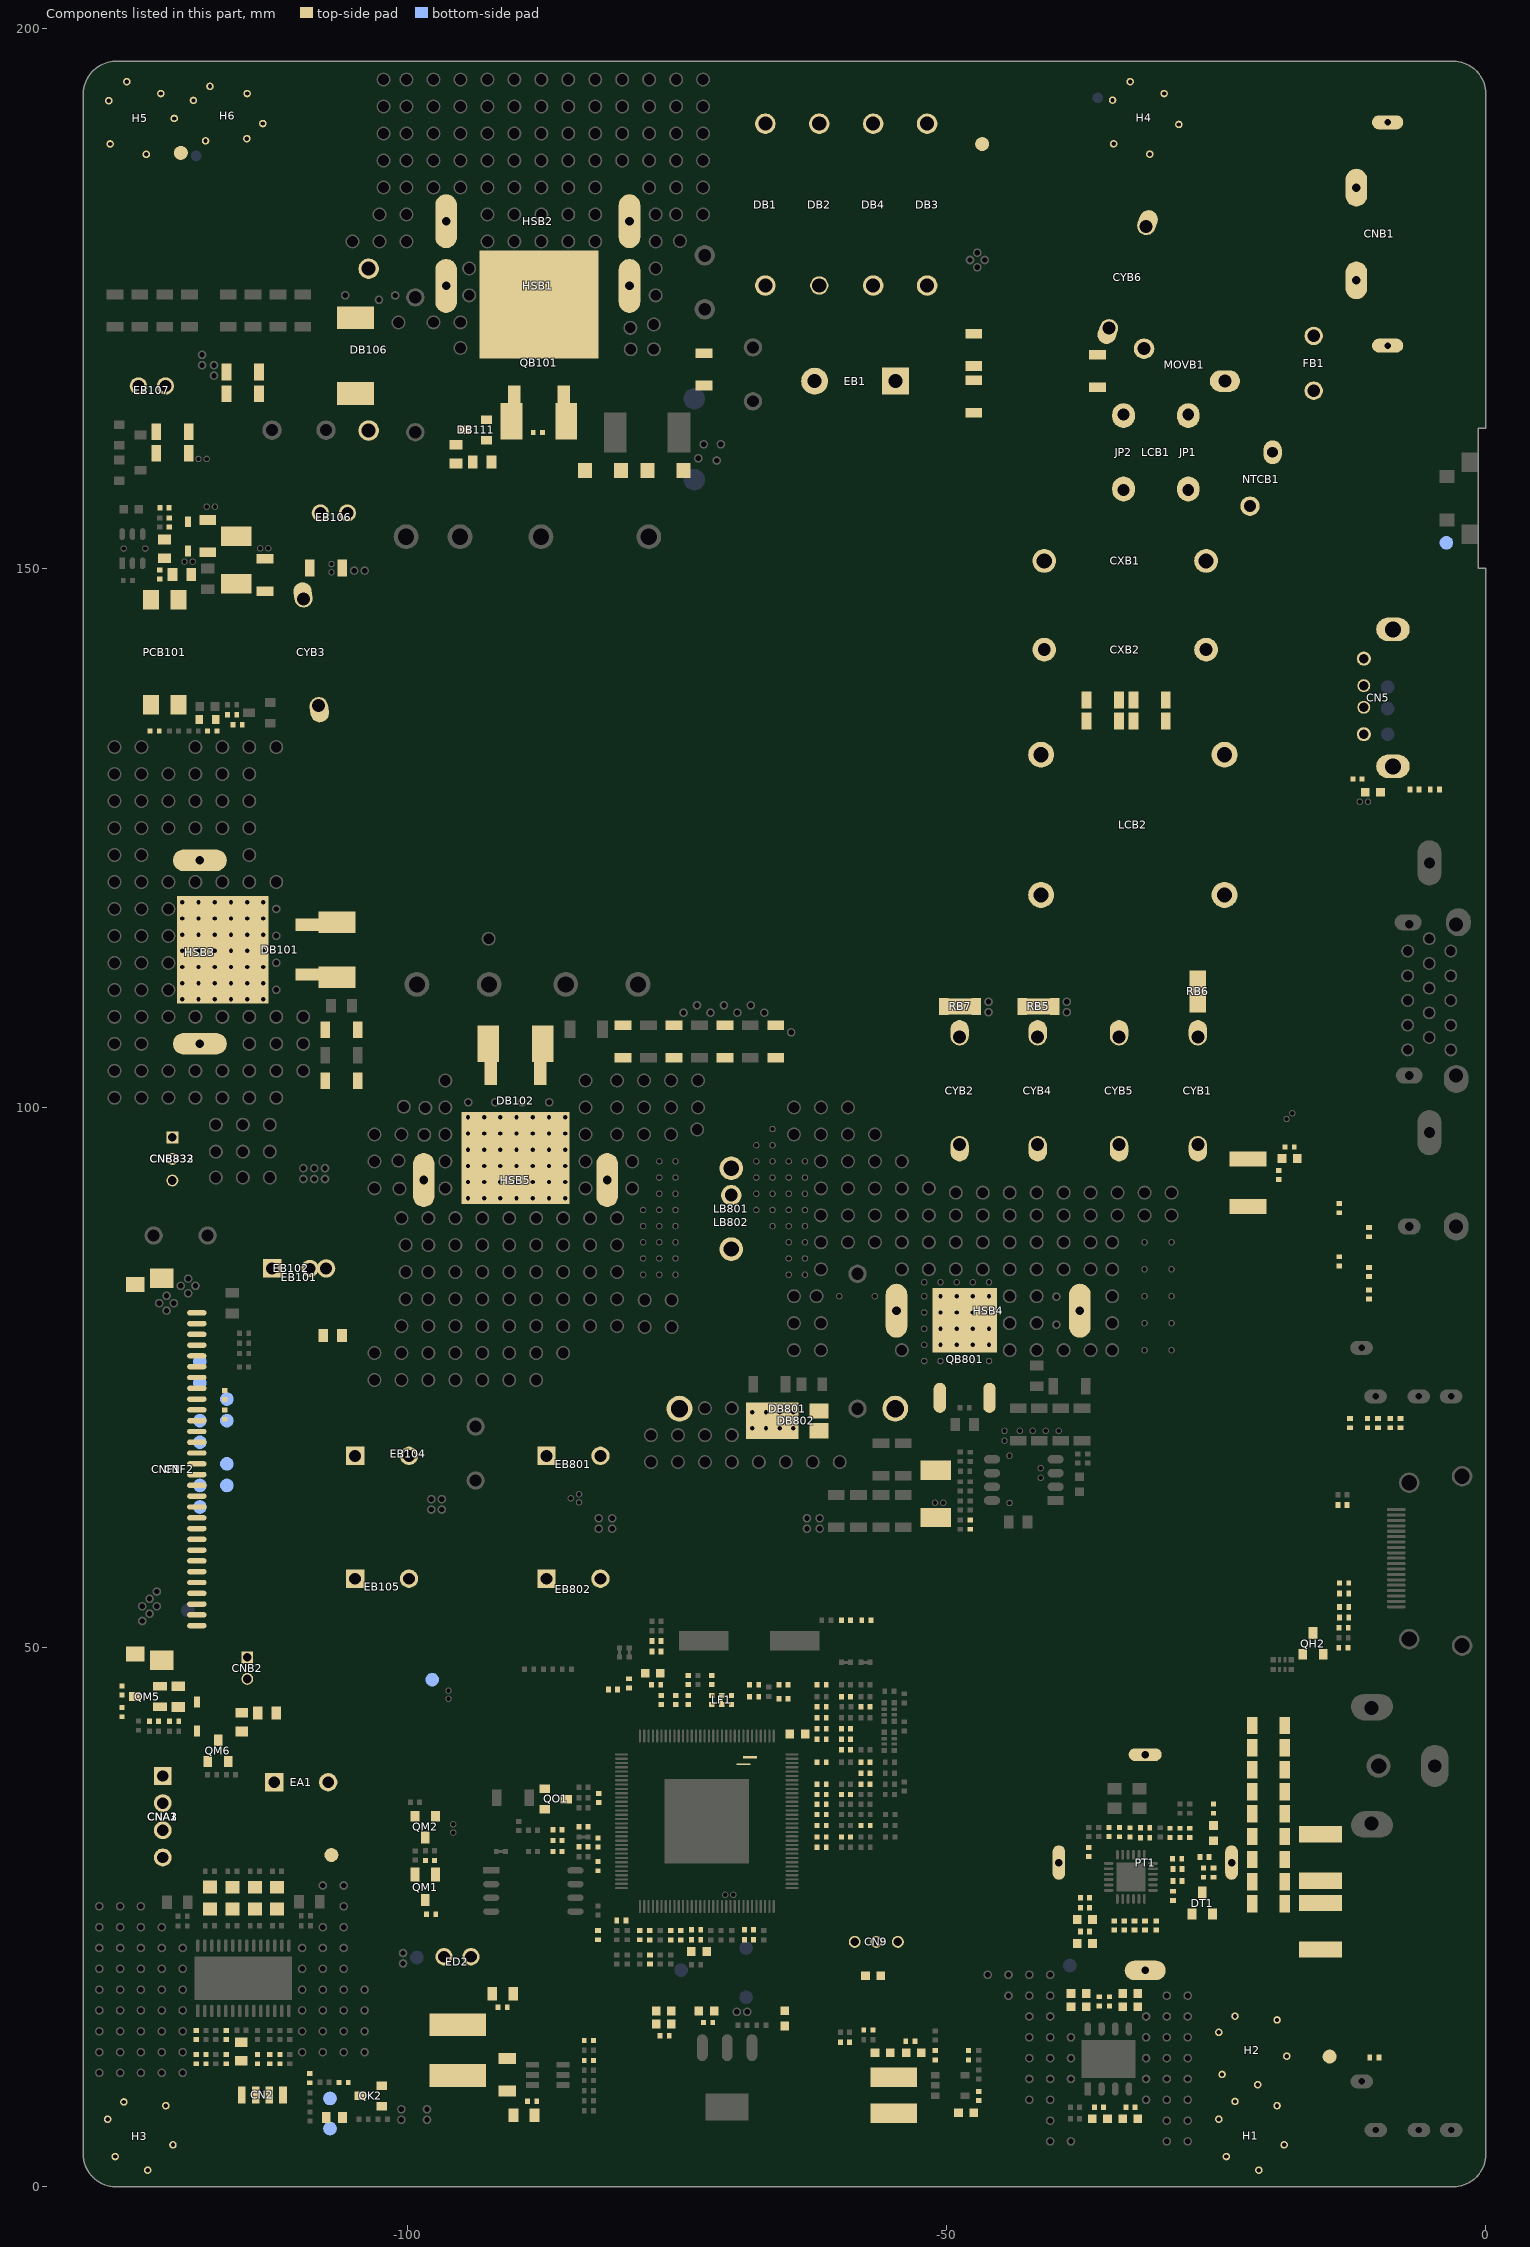
[diagram p0: the components of this part, seen from the top]
# Altium PCB MISC84438.PcbDoc (part 2 of 15)
Units mm, origin at the board's own origin, x right, y up, seen from the top; angles counter-clockwise.
Board outline 130 x 197 mm, 2 copper layers (TopLayer, BottomLayer), stack 1.571 mm thick; 574 components, 314 nets, 2636 pads, 811 vias.

## Components (designator, comment, footprint, x,y, rotation, side; value= is the part's Value field where it differs from the comment) (continued)
CB813 "100pF-0402-NPO-±5%-50V" C0402 -47.803,61.366 r90 top
CD1 "10uF-0805-X5R-±20%-16V" C0805 -89.154,6.629 r0 top
CD2 "0.1uF-0402-X5R-±20%-16V" C0402 -83.146,13.551 r0 top
CD11 "10uF-0603-X5R-±20%-6.3V" C0603 -48.171,6.858 r0 top
CD12 "NC/0.1uF-0402-X5R-±20%-16V" C0402 -47.015,8.395 r90 top
CD13 "3300pF-0402-X7R-±10%-50V" C0402 -47.955,12.179 r270 top
CD14 "10uF-0603-X5R-±20%-6.3V" C0603 -53.027,12.421 r180 top
CD15 "10uF-0603-X5R-±20%-6.3V" C0603 -55.918,12.408 r0 top
CD16 "NC/0.1uF-0402-X5R-±20%-16V" C0402 -53.34,13.487 r180 top
CD17 "Ceramic capacitor,CAP MC,6.3V,1uF,±20%,X5R,0402,SMD,TP" C0402 -51.027,12.179 r270 top
CD19 "NC/0.1uF-0402-X5R-±20%-16V" C0402 -88.392,7.925 r0 top
CD20 "NC/22pF-0402-NPO-±5%-50V" C0402 -83.146,11.697 r180 top
CD21 "NC/0.1uF-0402-X5R-±20%-16V" C0402 -91.135,16.612 r0 top
CD22 "10uF-0805-X5R-±20%-16V" C0805 -91.123,17.894 r0 top
CD41 "NC/10uF-1206-X5R-±10%-16V" C1206 -90.715,10.377 r270 top
CF1 "33pF-0402-NPO-±5%-50V" C0402 -73.939,46.964 r270 top
CF2 "0.1uF-0402-X5R-±20%-16V" C0402 -86.055,31.064 r0 top
CF4 "33pF-0402-NPO-±5%-50V" C0402 -71.755,46.964 r90 top
CF5 "10uF-0603-X5R-±20%-6.3V" C0603 -56.794,19.558 r0 top
CF6 "0.1uF-0402-X5R-±20%-16V" C0402 -82.22,36.017 r270 top
CF7 "0.1uF-0402-X5R-±20%-16V" C0402 -74.612,23.302 r90 top
CF8 "0.1uF-0402-X5R-±20%-16V" C0402 -61.57,31.445 r180 top
CF9 "0.1uF-0402-X5R-±20%-16V" C0402 -76.429,45.11 r270 top
CF10 "0.1uF-0402-X5R-±20%-16V" C0402 -61.57,36.347 r180 top
CF12 "0.1uF-0402-X5R-±20%-16V" C0402 -71.755,45.11 r270 top
CF13 "0.1uF-0402-X5R-±20%-16V" C0402 -61.57,39.344 r180 top
CF14 "0.1uF-0402-X5R-±20%-16V" C0402 -69.926,45.11 r270 top
CF15 "NC/10uF-0603-X5R-±20%-6.3V" C0603 -77.216,47.574 r180 top
CF16 "0.1uF-0402-X5R-±20%-16V" C0402 -76.911,46.507 r0 top
CF17 "0.1uF-0402-X5R-±20%-16V" C0402 -68.301,23.81 r180 top
CF18 "0.1uF-0402-X5R-±20%-16V" C0402 -78.435,23.314 r90 top
CF19 "0.1uF-0402-X5R-±20%-16V" C0402 -73.939,45.11 r270 top
CF20 "0.1uF-0402-X5R-±20%-16V" C0402 -82.296,29.705 r90 top
CF21 "0.1uF-0402-X5R-±20%-16V" C0402 -75.552,23.302 r90 top
CF22 "10uF-0603-X5R-±20%-6.3V" C0603 -72.936,21.79 r0 top
CF23 "Ceramic capacitor,CAP MC,6.3V,2.2uF,±20%,X5R,0402,SMD,TP" C0402 -75.082,45.11 r270 top
CF24 "0.1uF-0402-X5R-±20%-16V" C0402 -73.203,23.81 r180 top
CF25 "0.1uF-0402-X5R-±20%-16V" C0402 -73.203,22.872 r180 top
CF26 "0.047uF-0402-X7R-±10%-16V" C0402 -57.506,38.303 r0 top
CF28 "10uF-0603-X5R-±20%-6.3V" C0603 -63.805,41.961 r180 top
CF29 "NC/1000pF-0402-X7R-±10%-50V" C0402 -57.233,14.516 r0 top
CF30 "NC/1000pF-0402-X7R-±10%-50V" C0402 -59.405,13.398 r0 top
CF31 "NC/0.047uF-0402-X7R-±10%-16V" C0402 -57.48,33.477 r0 top
CF33 "NC/5pF-0402-NPO-±5%-50V" C0402 -116.896,71.552 r90 top
CF34 "NC/0.047uF-0402-X7R-±10%-16V" C0402 -61.57,37.312 r180 top
CF35 "NC/5pF-0402-NPO-±5%-50V" C0402 -116.896,73.381 r270 top
CF37 "10uF-0603-X5R-±20%-6.3V" C0603 -64.973,15.596 r270 top
CF38 "NC/0.1uF-0402-X5R-±20%-16V" C0402 -126.416,43.98 r270 top
CF39 "NC/NC/30pF-0402-NPO-±5%-50V" C0402 -59.309,52.489 r0 top
CF40 "Ceramic capacitor,CAP MC,50V,1000pF,±20%,X7R,0402,SMD,TP" C0402 -57.429,52.489 r180 top
CG1 "NC/0.1uF-0402-X5R-±20%-16V" C0402 -86.055,32.08 r180 top
CH8 "NC/0.1uF-0402-X5R-±20%-16V" C0402 -13.183,51.791 r0 top
CH9 "NC/0.1uF-0402-X5R-±20%-16V" C0402 -13.208,49.962 r0 top
CH10 "NC/30pF-0402-NPO-±5%-50V" C0402 -13.132,55.956 r180 top
CH15 "NC/1uF-0402-X5R-±20%-16V" C0402 -68.301,22.872 r180 top
CI1 "NC/0.047uF-0402-X7R-±10%-16V" C0402 -59.309,36.347 r0 top
CI3 "NC/0.1uF-0402-X5R-±20%-16V" C0402 -61.57,42.431 r0 top
CI4 "NC/0.1uF-0402-X5R-±20%-16V" C0402 -59.309,42.431 r0 top
CI6 "0.1uF-0402-X5R-±20%-16V" C0402 -59.309,40.5 r0 top
CI7 "0.1uF-0402-X5R-±20%-16V" C0402 -59.309,41.452 r0 top
CI8 "0.047uF-0402-X7R-±10%-16V" C0402 -57.506,37.313 r0 top
CI10 "NC/4700pF-0402-X7R-±10%-50V" C0402 -10.973,70.764 r90 top
CI11 "NC/4700pF-0402-X7R-±10%-50V" C0402 -8.865,70.764 r90 top
CK2 "0.01uF-0402-X7R-±10%-50V" C0402 -77.483,23.302 r270 top
CK4 "0.1uF-0402-X5R-±20%-16V" C0402 -109.004,10.058 r90 top
CK6 "NC/10pF-0402-NPO-±5%-50V" C0402 -83.642,31.496 r0 top
CK10 "NC/0.1uF-0402-X5R-±20%-16V" C0402 -105.867,9.652 r180 top
CL1 "NC/10uF-0603-X5R-±20%-6.3V" C0603 -72.238,16.281 r0 top
CL2 "0.1uF-0402-X5R-±20%-16V" C0402 -72.085,15.215 r0 top
CL3 "Ceramic capacitor,CAP MC,6.3V,1uF,±20%,X5R,0402,SMD,TP" C0402 -76.117,14.002 r0 top
CL4 "NC/10uF-0603-X5R-±20%-6.3V" C0603 -76.203,16.281 r0 top
CL5 "NC/10uF-0603-X5R-±20%-6.3V" C0603 -76.203,15.07 r0 top
CL6 "0.1uF-0402-X5R-±20%-16V" C0402 -35.852,7.366 r0 top
CL7 "NC/10uF-0603-X5R-±20%-6.3V" C0603 -35.776,6.299 r0 top
CL8 "NC/10uF-0603-X5R-±20%-6.3V" C0603 -32.956,6.299 r180 top
CL9 "0.1uF-0402-X5R-±20%-16V" C0402 -32.931,7.366 r180 top
CL10 "NC/0.1uF-0402-X5R-±20%-16V" C0402 -35.827,17.17 r270 top
CL11 "10uF-0603-X5R-±20%-6.3V" C0603 -37.744,17.907 r180 top
CL12 "NC/10uF-0603-X5R-±20%-6.3V" C0603 -37.744,16.688 r180 top
CL13 "NC/0.1uF-0402-X5R-±20%-16V" C0402 -34.887,17.17 r90 top
CL14 "10uF-0603-X5R-±20%-6.3V" C0603 -32.956,16.688 r0 top
CL15 "NC/10uF-0603-X5R-±20%-6.3V" C0603 -32.956,17.907 r180 top
CM1 "0.22uF-0402-X5R-±10%-16V" C0402 -97.866,30.233 r0 top
CM2 "0.1uF-0402-X5R-±20%-16V" C0402 -97.765,25.248 r180 top
CM3 "NC/0.1uF-0402-X5R-±20%-16V" C0402 -121.577,43.142 r0 top
CM4 "0.1uF-0402-X5R-±20%-16V" C0402 -126.416,45.987 r90 top
CM5 "NC/10uF-0805-X5R-±20%-16V" C0805 -121.196,45.428 r90 top
CM7 "0.022uF-0402-X7R-±10%-16V" C0402 -123.457,43.142 r180 top
CN2 "IR receiver transistor,IR Receriver,2.7-5.5V,37.9KHz,SMD,SIRAB39,SL" REMOTE-HS-1 -113.4,6.227 r0 top locked
CN5 "USB terminal,USB Jack,USB2.0,H,Single,Black,flange,Block up,DIP,103411481,VAST" USB-HD-30 -0.5,138 r90 top locked
CN9 "NC/Connector socket,connect jack,3Pin,D2.0,D,SNAP,Nature,L=2.8mm,DIP,AMA" SIP3/2.0D-3 -56.5,22.687 r0 top
CNA1 "NC/4PIN-2.54-D-H-G" SIP4/2.54D-1 -122.636,34.29 r270 top locked
CNA2 "Connector socket,connect jack,4PIN,D2.50,L,SNAP,STEP,Fool-proofing,Nature,L=3.0mm,DIP,AMA" SIP4H/2.54D-2 -122.636,34.29 r270 top locked
CNA3 "NC/Connector socket,connect jack,4Pin,D2.50,D,SNAP,nature,L=2.8mm,DIP,CNJST" SIP4/2.5D-2 -122.636,34.29 r270 top locked
CNB1 "Red-phosphorus-free connector socket,connect jack(HP),2Pin,D8.6,L,SNAP,Fool-proofing,Black,L=4.0mm,DIP,YQ" CON2-H8.6-1 -12.5,181 r90 top locked
CNB2 "Connector socket,connect jack,2Pin,D2.0,D,Beige,L=2.8mm,DIP,W2011-02SVA-SN8-ENSY,XYDT" SIP2/2.0D-1 -114.808,48.057 r270 top
CNB832 "NC/Connector socket,connect jack,3Pin,D2.0,D,SNAP,L=2.8mm,DIP,CNJST" SIP3/2.0D-CP -121.744,95.263 r270 top
CNB833 "Connector socket,connect jack,3Pin,D2.0,L,SNAP,STEP,Nature,L=2.8mm,DIP,AMA" SIP3H/2.0D-3 -121.744,95.263 r270 top
CNF1 "NC/FFC socket,FFC connector,30Pin,D1.0,Bottom,lock,SMD,F10033FA030M1WL,CT" FFC30H/1.0S-7 -122.333,66.5 r270 top
CNF2 "FFC socket,FFC connector,30Pin,D1.0,Bottom,SMD,P-TWO" FFC30H/1.0S-1 -121.111,66.5 r270 top locked
CO1 "1uF-0402-X5R-±20%-6.3V" C0402 -57.506,44.475 r0 top
CO3 "NC/1000pF-0402-X7R-±10%-50V" C0402 -61.57,43.459 r180 top
CO4 "1uF-0402-X5R-±20%-6.3V" C0402 -59.309,45.415 r180 top
CO5 "NC/1000pF-0402-X7R-±10%-50V" C0402 -61.57,44.475 r180 top
CO9 "100pF-0402-NPO-±5%-50V" C0402 -57.506,39.344 r180 top
COLD "COLD" COLD -15.494,75.794 r90 top
"Conformal Coating" "NC/Conformal coating,25kg/Can,Peters" "Conformal Coating" -147.574,131.394 r90 top
CQC "CQC" CQC -106.401,47.625 r270 top
CT1 "0.1uF-0402-X5R-±20%-16V" C0402 -36.805,31.013 r90 top
CT3 "NC/10uF-0603-X5R-±20%-6.3V" C0603 -37.16,22.543 r0 top
CT5 "0.1uF-0402-X5R-±20%-16V" C0402 -37.16,25.845 r0 top
CT6 "10uF-0603-X5R-±20%-6.3V" C0603 -37.16,24.765 r180 top
CT7 "33pF-0402-NPO-±5%-50V" C0402 -28.346,32.791 r270 top
CT8 "33pF-0402-NPO-±5%-50V" C0402 -27.432,32.791 r270 top
CT9 "0.1uF-0402-X5R-±20%-16V" C0402 -30.543,24.206 r270 top
CT10 "33pF-0402-NPO-±5%-50V" C0402 -65.107,45.212 r0 top
CT11 "0.022uF-0402-X7R-±10%-16V" C0402 -33.533,24.206 r90 top
CT12 "0.022uF-0402-X7R-±10%-16V" C0402 -34.461,24.206 r270 top
CT13 "NC/1.2pF-0402-NPO-±0.25pf-50V" C0402 -26.167,29.103 r270 top
CT14 "NC/8pF-0402-NPO-±5%-50V" C0402 -34.925,32.88 r90 top
CT15 "NC/8pF-0402-NPO-±5%-50V" C0402 -33.96,32.854 r270 top
CT17 "NC/180pF-0402-NPO-±5%-50V" C0402 -25.248,35.039 r90 top
CT18 "0.1uF-0402-X5R-±20%-16V" C0402 -37.16,26.772 r0 top
CT19 "0.022uF-0402-X7R-±10%-16V" C0402 -61.57,46.507 r180 top
CT20 "0.1uF-0402-X5R-±20%-16V" C0402 -67.825,45.415 r180 top
CT21 "0.047uF-0402-X7R-±10%-16V" C0402 -28.613,30.391 r0 top
CT23 "0.1uF-0402-X5R-±20%-16V" C0402 -67.825,46.507 r180 top
CT24 "33pF-0402-NPO-±5%-50V" C0402 -65.107,46.507 r180 top
CT25 "0.1uF-0402-X5R-±20%-16V" C0402 -29.273,32.791 r90 top
CT26 "330pF-0402-NPO-±5%-50V" C0402 -31.572,32.346 r0 top
CT27 "0.1uF-0402-X5R-±20%-16V" C0402 -32.982,32.842 r90 top
CT29 "6800pF-0402-X7R-±10%-50V" C0402 -31.572,33.274 r0 top
CT40 "Ceramic capacitor,CAP MC,1KV,470pF,±5%,NPO,1206,SMD,TP" C1206 -20.142,32.448 r180 top
CT41 "4700pF-1206-X7R-±10%-1000V" C1206 -20.142,34.569 r0 top
CT42 "4700pF-1206-X7R-±10%-1000V" C1206 -20.142,30.328 r0 top
CT43 "4700pF-1206-X7R-±10%-1000V" C1206 -20.142,28.27 r0 top
CT44 "4700pF-1206-X7R-±10%-1000V" C1206 -20.142,36.601 r0 top
CT45 "4700pF-1206-X7R-±10%-1000V" C1206 -20.142,26.213 r0 top
CT46 "4700pF-1206-X7R-±10%-1000V" C1206 -20.142,38.633 r0 top
CT47 "NC/4700pF-1206-X7R-±10%-1000V" C1206 -20.142,42.746 r0 top
CT48 "4700pF-1206-X7R-±10%-1000V" C1206 -20.142,40.691 r0 top
CU1 "NC/10uF-0603-X5R-±20%-6.3V" C0603 -10.465,129.261 r180 top
CU2 "Ceramic capacitor,CAP MC,6.3V,0.47uF,±10%,X5R,0402,SMD,TP" C0402 -11.887,130.48 r180 top
CU3 "NC/Ceramic capacitor,CAP MC,6.3V,0.47uF,±10%,X5R,0402,SMD,TP" C0402 -18.186,96.368 r0 top
CU4 "NC/10uF-0603-X5R-±20%-6.3V" C0603 -18.186,95.301 r180 top
CV1 "NC/0.047uF-0402-X7R-±10%-16V" C0402 -61.57,34.493 r0 top
CV3 "NC/0.047uF-0402-X7R-±10%-16V" C0402 -61.57,33.477 r0 top
CV7 "NC/0.047uF-0402-X7R-±10%-16V" C0402 -59.309,32.41 r0 top
CV9 "NC/33pF-0402-NPO-±5%-50V" C0402 -61.57,32.41 r180 top
CV10 "NC/33pF-0402-NPO-±5%-50V" C0402 -61.57,35.433 r180 top
CXB1 "X capacitor,CAP X2,MP,275VAC,0.47uF,±10%,S,15mm-Mini,PC,DIP,BM" CAP18*8.5-V-15 -33.432,150.692 r180 top locked
CXB2 "NC/X capacitor,CAP X2,MP,280VAC,0.1uF,±10%,P,15mm,PC,DIP,JH" CAP18*5*11.5-V-15 -33.432,142.471 r0 top
CYB1 "Y capacitor,CAP Y1,CD,470pF,400VAC,±20%,KS,10mm,Y5U,DIP,Walsin" CAP13*5-V-10-1 -26.691,101.582 r270 top locked
CYB2 "Y capacitor,CAP Y1,CD,470pF,400VAC,±20%,KS,10mm,Y5U,DIP,Walsin" CAP13*5-V-10-1 -48.777,101.582 r270 top
CYB3 "Y capacitor,CAP Y1,CD,470pF,400VAC,±20%,KS,10mm,Y5U,DIP,Walsin" CAP13*5-V-10-1 -108.882,142.227 r278 top locked
CYB4 "NC/Y capacitor,CAP Y1,CD,47pF,400VAC,±5%,KS,10mm,SL,DIP,BULK,Walsin" CAP13*5-V-10-1 -41.538,101.582 r270 top locked
CYB5 "NC/Y capacitor,CAP Y1,CD,47pF,400VAC,±5%,KS,10mm,SL,DIP,BULK,Walsin" CAP13*5-V-10-1 -33.994,101.582 r270 top locked
CYB6 "Y capacitor,CAP Y1,CD,100pF,400VAC,±10%,KS,10mm,Y5P,DIP,Walsin" CAP13*5-V-10-1 -33.2,177 r70 top
DB1 "Rectifier diode,DIO SI S,2.5A,1000V,DO-15,DIP,RL257G,YJ" D2-H-15#1 -66.788,183.722 r90 top locked
DB2 "Rectifier diode,DIO SI S,2.5A,1000V,DO-15,DIP,RL257G,YJ" D2-H-15#2 -61.788,183.722 r270 top locked
DB3 "Rectifier diode,DIO SI S,2.5A,1000V,DO-15,DIP,RL257G,YJ" D2-H-15#3 -51.788,183.722 r90 top locked
DB4 "Rectifier diode,DIO SI S,2.5A,1000V,DO-15,DIP,RL257G,YJ" D2-H-15#4 -56.788,183.722 r270 top locked
DB101 "Schottky diode,DIO SBD D1,10A,150V,TO-263,SMD,HBR10150SS,JLHW" D2PAK3#1 -117.091,114.655 r90 top locked
DB102 "Schottky diode,DIO SBD D1,10A,200V,TO-263,SMD,HBR10200SS,JLHW" D2PAK3#1 -89.948,95.345 r180 top
DB103 "NC/Rectifier diode,DIO SI S,3A,1000V,SMC,SMD,HS3M R6,TSC" DIODE-SMC -104.775,169.723 r90 top locked
DB104 "Rectifier diode,DIO SI S,1A,1000V,SMAF,SMD,M7F,YJ" DIODE-S-2 -115.83,150.795 r90 top
DB106 "Rectifier diode,DIO FRD S,2A,1000V,DO-15,DIP,FR207G-FG-WS,WILLAS" D2-H-15#5 -103.554,170.282 r270 top
DB109 "Rectifier diode,DIO FRD S,1.2A,800V,SOD-123FL,SMD,F1K,YJ" DIODE-S-14 -81.842,159.075 r180 top
DB110 "Rectifier diode,DIO FRD S,1.2A,800V,SOD-123FL,SMD,F1K,YJ" DIODE-S-14 -76.028,159.075 r180 top
DB111 "Switching diode,DIO SW D1,215mA,85V,SOT-23,SMD,KAV70,KEXIN" SO-23 -93.637,162.839 r270 top
DB112 "NC/Switching diode,DIO SW S,200mA,250V,SOD-323,SMD,BAV21WS,BLUE ROCKET" DIODE-S-12 -120.307,152.971 r270 top
DB801 "Schottky diode,DIO SBD S,3A,100V,DO-201AD,DIP,SR3100,YJ" D3-H-20-2 -64.742,72.114 r180 top
DB802 "NC/TSPB5H150S" DIODE-S-13 -64.734,70.989 r90 top
DB804 "Rectifier diode,DIO SI S,1A,1000V,SMAF,SMD,M7F,YJ" DIODE-S-2 -50.99,64.224 r270 top
DH2 "NC/0ohm-0402-±5%-1/16W" DIODE-S0402 -13.284,63.195 r0 top
DH3 "NC/NC/AVLC18S02003" DIODE-S0402 -13.132,54.991 r0 top
DH6 "NC/NC/AVLC18S02003" DIODE-S0402 -13.132,53.746 r0 top
DH7 "NC/NC/AVLC18S02003" DIODE-S0402 -13.132,52.756 r0 top
DH8 "NC/NC/AVLC18S02003" DIODE-S0402 -80.137,24.689 r0 top
DH9 "NC/NC/AVLC18S02003" DIODE-S0402 -82.296,23.314 r90 top
DI1 "NC/AVLC18S02003" DIODE-S0402 -10.82,82.702 r90 top
DI2 "NC/AVLC18S02003" DIODE-S0402 -10.82,88.468 r90 top
DI3 "NC/AVLC18S02003" DIODE-S0402 -13.589,90.703 r90 top
DI5 "NC/AVLC18S02003" DIODE-S0402 -10.338,11.989 r180 top
DK1 "TVS diode,DIO ESD,3pF,58V,0402,SMD,SDV1005H260C030YPTF,Sunlord" DIODE-S0402 -77.495,21.054 r270 top
DK20 "WEJT61RC-871-red" DIODE-S0603 -106.73,6.417 r0 top locked
DM1 "NC/Switching diode,DIO SW S,150mA,75V,SOD-323,SMD,1N4148WS,BLUE ROCKET" DIODE-S-12 -119.456,43.586 r90 top
DO1 "NC/AVLC18S02003" DIODE-S0402 -10.008,70.764 r90 top
DO2 "NC/AVLC18S02003" DIODE-S0402 -12.573,70.764 r90 top
DO3 "NC/AVLC18S02003" DIODE-S0402 -7.899,70.764 r90 top
DT1 "Switching diode,DIO SW D2,75V,SOT-23,SMD,KAV99,KEXIN" SO-23 -26.289,26.289 r180 top
DT2 "NC/AVLC18S02003" DIODE-S0402 -76.879,50.569 r0 top
DT3 "NC/AVLC18S02003" DIODE-S0402 -76.879,49.603 r0 top
DU1 "NC/" DIODE-S0402 -80.899,46.101 r0 top
DU2 "NC/" DIODE-S0402 -79.426,46.66 r270 top
DU3 "NC/" DIODE-S0402 -6.604,129.488 r0 top
DU4 "NC/" DIODE-S0402 -4.724,129.488 r180 top
DV1 "NC/NC/AVLC18S02003" DIODE-S0402 -13.589,85.776 r90 top
DV2 "NC/NC/AVLC18S02003" DIODE-S0402 -10.82,84.785 r90 top
E0N "TEST" TP -119.2,63 r180 bottom
E0P "TEST" TP -119.2,65 r180 bottom
E1N "TEST" TP -116.7,65 r180 bottom
E1P "TEST" TP -116.7,67 r180 bottom
E2N "TEST" TP -119.2,69 r180 bottom
E2P "TEST" TP -119.2,71 r180 bottom
E3N "TEST" TP -119.2,74.5 r180 bottom
E3P "TEST" TP -119.2,76.5 r180 bottom
EA1 "Aluminum electrolytic capacitor,CAP AL,16V,470uF,±20%,KM,P,5.0mm,10×12.5,DIP,TP,Samxon" EC(10*12.5)-V-5#1 -109.804,37.486 r0 top locked
EB1 "Aluminum electrolytic capacitor,CAP AL,450V,82uF,±20%,SL,KL,BK,7.5mm,18×35.5,DIP,CapXon" EC(18*41)-H-7.5-1 -58.458,164.859 r0 top locked
EB101 "Aluminum electrolytic capacitor,CAP AL,25V,470uF,±20%,LD,GK,P,5.0mm,10×12.5,DIP,TP,Samxon" EC(10*12.5)-V-5#2 -110,85.114 r0 top locked
EB102 "NC/270uF-16V-±20%-8×11-105℃-RP-short leg-F=3.5(Elite)" EC(8*11)-V-3.5 -110.75,85.114 r0 top locked
EB104 "Aluminum electrolytic capacitor,CAP AL,63V,100uF,±20%,LD,GF,P,5.0mm,10×12.5,DIP,TP,CapXon" EC(10*12.5)-V-5#3 -102.311,67.742 r0 top locked
EB105 "Aluminum electrolytic capacitor,CAP AL,63V,100uF,±20%,LD,GF,P,5.0mm,10×12.5,DIP,TP,CapXon" EC(10*12.5)-V-5#4 -102.311,56.35 r0 top locked
EB106 "Aluminum electrolytic capacitor,CAP AL,50V,10uF,±20%,LF,GH,P,2.5mm,5×11,DIP,TP,CapXon" EC(5*11)-V-2.5#1 -106.782,155.138 r0 top locked
EB107 "NC/Aluminum electrolytic capacitor,CAP AL,50V,4.7uF,±20%,LC,LL,P,2.5mm,5×11,DIP,TP,CapXon" EC(5*11)-V-2.5#2 -123.652,166.916 r0 top locked
EB801 "Aluminum electrolytic capacitor,CAP AL,100V,47uF,±20%,LD,SF,P,5.0mm,10×12.5,DIP,TP,Samxon" EC(10*12.5)-V-5#5 -84.573,67.742 r0 top locked
EB802 "NC/47uF-100V-±20%-10×12-105℃-EV-taped reel-F=5.0(Elite)" EC(10*12.5)-V-5#6 -84.573,56.35 r0 top locked
ECN "TEST" TP -116.7,71 r180 bottom
ECP "TEST" TP -116.7,73 r180 bottom
ED2 "Aluminum electrolytic capacitor,CAP AL,10V,470uF,±20%,KM,P,2.5mm,6.3×11.0,DIP,TP,Samxon" EC(6.3*11)-V-2.5 -95.326,21.311 r0 top locked
F1 "NC/MSMD110" FUSE3.5A-S -22.041,93.059 r270 top
F2 "0ohm-0402-±5%-1/16W" R0402 -19.196,93.777 r90 top
FB1 "Slow-blow fuse,FUSE T,P,3.15A,250VAC,8.5×4.0×8mm,DIP,TP,Walter" "FUSE8.5*4-V-5(T3.15AL 250V~)" -15.953,169.012 r90 top
GDT1 "NC/Gas discharge tube,GDT,700V,2000A,TP,4.5*3.2mm,SMD,4532-091-LF,Brightking" SMD4532-1 -15.316,30.505 r270 top
GDT2 "NC/Gas discharge tube,GDT,700V,2000A,TP,4.5*3.2mm,SMD,4532-091-LF,Brightking" SMD4532-1 -15.316,24.143 r90 top
GL1 "Silicone,0.5g,general,60,white,SLD-8854W,XY" "Silica gel-20" -48.006,132.461 r180 top
H1 "Location hole" ASSE4.0C-3#1 -22,5 r0 top locked
H2 "Location hole" ASSE4.0C-3#2 -22,13 r0 top locked
H3 "Location hole" ASSE4.0C-3#3 -125,5 r0 top locked
H4 "Location hole" ASSE4.0C-3#4 -32,192 r0 top locked
H5 "Location hole" ASSE4.0C-3#5 -125,192 r0 top locked
H6 "Location hole" ASSE4.0C-3#6 -117,192 r0 top locked
"High Voltage" "High Voltage" "High Voltage" -21.59,177.971 r0 top
HOT "HOT" HOT -38.964,113.64 r0 top
HS1 "Heatsink,6-series aluminium alloy,14.0×14.0×6.0mm,natural colour,XXWJ" HS(14*14*6) -72.212,33.871 r0 top locked
HSB1 "NC/17.5×14.5×0.5- natural finish -Cu-MRD" HS038 -87.874,176.188 r180 top
HSB2 "NC/17.5×14.5×0.5- natural finish -Cu-MRD" HS038 -87.874,182.188 r180 top
HSB3 "NC/17.5×14.5×0.5- natural finish -Cu-MRD" HS038 -119.2,114.438 r270 top
HSB4 "NC/17.5×14.5×0.5- natural finish -Cu-MRD" HS038 -46.126,81.193 r0 top
HSB5 "NC/17.5×14.5×0.5- natural finish -Cu-MRD" HS038 -89.948,93.305 r180 top
IR "TEST" TP -107.137,5.385 r180 bottom
JP1 "NC/Jumper,RES JUMP,0.6,7.0mm,DIP" JP7.0#1 -27.582,160.763 r90 top locked
JP2 "NC/Jumper,RES JUMP,0.6,7.0mm,DIP" JP7.0#2 -33.582,160.763 r90 top locked
KEY "TEST" TP -3.658,152.375 r180 bottom
LB801 "Differential-mode inductor,Inductor,DR12×12,70uH,0.15×12P,38.5Ts,H13.5MAX,SYDR1212-L070uA,DIP,DL" L/LC2/15*14.5-V7.5 -69.946,90.65 r90 top locked
LB802 "NC/Differential-mode inductor,Inductor,DR12×14,68uH,0.45,20Ts,H13.5MAX,SYDR1214-L068uA,DIP,Soldier" L(13.5*15.5)-V-5 -69.945,89.4 r90 top locked
LBA1 "Ferrite bead,BEAD,300ohm,0805,3000mA,SMD,TP,HCB2012KF-301T30,Tai-tech" L0805 -118.274,26.759 r90 top
LBA2 "Ferrite bead,BEAD,300ohm,0805,3000mA,SMD,TP,HCB2012KF-301T30,Tai-tech" L0805 -116.191,26.733 r90 top
LBA3 "Ferrite bead,BEAD,300ohm,0805,3000mA,SMD,TP,HCB2012KF-301T30,Tai-tech" L0805 -114.108,26.733 r90 top
LBA4 "Ferrite bead,BEAD,300ohm,0805,3000mA,SMD,TP,HCB2012KF-301T30,Tai-tech" L0805 -112.051,26.733 r90 top
LCB1 "Common-mode choke,Common Choke,T9×5×3,230uH MIN,0.45×1P,7.5Ts,H14.0MAX,SYT09-L230uA,DIP,CK" L/LC4/12.8*10-V-6*7 -30.582,160.763 r180 top locked
LCB2 "Common-mode choke,Common Choke,UC1614,10.5mH±10%,0.15×1.0mm,48Ts,H14.0MAX,SYUC16-L10.5mA,DIP,CH" L/LC4/21*17-H-17*13 -32.722,126.231 r180 top locked
LD2 "Power inductor,Power Inductor,6.8uH,±20%,1.3A,0.23×1P,DR4.5×3.2,SMD,DSB4532-6R8M-LF,BLDX" L(4.5*3.5)-S -54.864,8.471 r90 top
LD3 "Power inductor,Power Inductor,4.7uH,±20%,2.8A,0.32×1P,DR5.8×4.5,SMD,PIO54-4R7MTP02,FH" L(6.0*4.5)-S -95.301,12.649 r90 top
LED "TEST" TP -107.137,8.179 r180 bottom
LF1 "NC/0ohm-0402-PCB" R0402SC -70.841,45.11 r90 top
LF6 "0ohm-0402-±5%-1/16W" R0402 -61.57,41.453 r180 top
LT1 "Multilayer inductor,HF Inductor,68nH,±5%,0402,SMD,SDCL1005C68NJTDF,Sunlord" L0402 -31.61,24.206 r90 top
LT2 "GZ1005U102CTF(1000ohm-300mA)" L0402 -32.575,24.206 r270 top
LT3 "0ohm-0402-±5%-1/16W" L0402 -25.227,29.103 r270 top
LT6 "GZ1005U102CTF(1000ohm-300mA)" L0402 -28.981,26.962 r270 top
LT8 "GZ1005U102CTF(1000ohm-300mA)" L0402 -28.588,28.32 r0 top
LT9 "NC/SDCL1608CR22JT(F)" L0603 -25.248,32.779 r90 top
LT10 "SDCL1005CR18JTDF(180nH-0402±5%-C)" L0402 -28.588,29.425 r0 top
LT11 "NC/SDCL1005CR27JTDF (Sunlord)" L0402 -26.086,30.556 r180 top
LT12 "Ferrite bead,BEAD,120ohm,0402,500mA,SMD,TP,GZ1005U121CTF,Sunlord" L0402 -37.16,23.66 r0 top
M1 "MARK" MARK -14.478,12.052 r0 top
M2 "MARK" MARK -107.01,30.734 r0 top
M3 "MARK" MARK -120.968,188.519 r0 top
M4 "MARK" MARK -46.685,189.332 r0 top
Manufacture_Info "Manufacture_Info" Manufacture_Info -73.4,33.6 r180 top
MOVB1 "Varistor,VARISTOR,128J,680V,4000A,S,7.5mm,10mm,DIP,Thinking" VR(13*5)-V-7.5 -27.932,168.866 r0 top
"NO DOLBY" "NO DOLBY" "NO DOLBY-SILK" -80.5,5.9 r0 bottom
NTCB1 "SCK102R55AMBY502 (short leg / Weiqin)" NTC(10*5)-V5 -20.812,158.268 r90 top
PCB101 "LTV-817S-TA-B (Lite-On)" OC4-S-1 -122.45,142.227 r0 top locked
PT1 "20.3×16.3×6-LHD (with sealing)" SHIELD(16*20*6) -31.572,20.041 r0 top locked
PWM_REF "NC/TEST" TP_BL -97.663,46.99 r90 bottom
QB101 "MOSFET,NMOS,7A,650V,0.55ohm@ID=3.5A@VGS=10V,TO-252,LSG65R650HT,LONTEN" D2PAK3#2 -87.871,171.12 r270 top
QB801 "MOSFET,NMOS,15A,100V,0.105ohm@ID=6A@VGS=10V,TO-252,PA110BDA,UNIKC" TO-252-GDS -48.311,80.315 r0 top locked
QH2 "LMBT3904LT1G" SOT-23 -16.027,50.368 r180 top
QK2 "NC/MMBT3904(f≥350MHz)" SOT-23 -103.365,8.407 r270 top
QM1 "MOSFET,PMOS,-4.2A,-30V,0.052ohm@ID=-4.2A@VGS=-10V,SOT23-3,AO3401,BLUE ROCKET" SOT-23-1 -98.311,27.731 r0 top
QM2 "MMBT3904(f≥350MHz)" SOT-23 -98.311,33.319 r0 top
QM5 "MOSFET,PMOS,-4.3A,-30V,0.078ohm@ID=-3A@VGS=-4.5V,SOT-23,AO3487,AOS" SOT-23-1 -124.092,45.428 r270 top
QM6 "MMBT3904(f≥350MHz)" SOT-23 -117.526,40.411 r180 top
QO1 "NC/MMBT3904(f≥350MHz)" SOT-23 -86.208,35.938 r90 top
R1 "4K7ohm-0402-±5%-1/16W" R0402 -83.642,33.35 r180 top
R2 "4K7ohm-0402-±5%-1/16W" R0402 -82.296,31.902 r90 top
R3 "NC/4K7ohm-0402-±5%-1/16W" R0402 -86.055,33.071 r180 top
R5V "NC/0ohm-0805-±5%-1/8W" R0805 -112.979,43.917 r180 top
R12V "0ohm-0805-±5%-1/8W" R0805 -115.316,43.053 r90 top
RA1 "4K7ohm-0402-±5%-1/16W" R0402 -119.544,11.822 r270 top
RA2 "NC/" GND#1 -68.223,39.802 r180 top
RA3 "10ohm-0805-±5%-1/8W" R0805 -115.367,12.522 r90 top
RA4 "NC/100Kohm-0402-±5%-1/16W" R0402 -116.737,11.822 r270 top
RA5 "1Kohm-0402-±5%-1/16W" R0402 -111.772,11.822 r90 top
RA8 "4K7ohm-0402-±5%-1/16W" R0402 -119.544,14.057 r90 top
RA11 "4K7ohm-0402-±5%-1/16W" R0402 -113.854,11.822 r90 top
RA12 "NC/3K3ohm-0402-±5%-1/16W" R0402 -112.737,11.822 r90 top
RA14 "NC/0ohm-0402-±5%-1/16W" R0402 -116.737,14.057 r90 top
RA15 "NC/" GND#2 -68.809,39.167 r180 top
RA21 "1Kohm-0402-±5%-1/16W" R0402 -118.629,11.822 r90 top
RB1 "1M2ohm-1206-±5%-1/4W" R1206 -31.168,137.812 r180 top
RB2 "1M2ohm-1206-±5%-1/4W" R1206 -31.168,135.851 r180 top
RB3 "1M2ohm-1206-±5%-1/4W" R1206 -35.511,137.811 r180 top
RB4 "1M2ohm-1206-±5%-1/4W" R1206 -35.511,135.849 r180 top
RB5 "NC/0ohm-1206-PCB-D" R1206SC -41.47,109.398 r180 top
RB6 "NC/0ohm-1206-PCB-D" R1206SC -26.7,110.8 r270 top
RB7 "NC/0ohm-1206-PCB-D" R1206SC -48.734,109.398 r180 top
RB8 "30ohm-1206-±5%-1/4W" R1206 -36,168.3 r90 top
RB101 "330Kohm-1206-±5%-1/4W" R1206 -47.473,170.256 r270 top
RB102 "330Kohm-1206-±5%-1/4W" R1206 -47.473,165.938 r270 top
RB103 "Thick-film resistor,RES,1/16W,3.6Kohm,±1%,0402,SMD" R0402 -122.022,154.254 r90 top
RB104 "Thick-film resistor,RES,1/16W,39Kohm,±1%,0402,SMD" R0402 -122.936,149.428 r270 top
RB105 "Thick-film resistor,RES,1/16W,510ohm,±1%,0402,SMD" R0402 -122.479,155.613 r0 top
RB106 "Thick-film resistor,RES,1/8W,68ohm,±5%,0805,SMD" R0805 -93.04,159.88 r0 top
RB107 "Thick-film resistor,RES,1/8W,20ohm,±5%,0805,SMD" R0805 -95.462,160.596 r90 top
RB109 "Thick-film resistor,RES,1/16W,10Kohm,±1%,0402,SMD" R0402 -87.871,162.598 r180 top
RB110 "0ohm-1206-±5%-1/4W" R1206 -121.742,160.68 r0 top
RB111 "0ohm-1206-±5%-1/4W" R1206 -121.742,162.655 r0 top
RB112 "NC/33Kohm-0805-±1%-1/8W" R0805 -122.479,151.816 r270 top
RB113 "Thick-film resistor,RES,1/8W,300Kohm,±1%,0805,SMD" R0805 -120.879,149.428 r0 top
RB114 "Thick-film resistor,RES,1/4W,4.7ohm,±1%,1206,SMD" R1206 -113.16,149.395 r90 top
RB116 "NC/10ohm-1206-±5%-1/4W" R1206 -118.478,152.984 r90 top
RB117 "Thick-film resistor,RES,1/4W,10ohm,±5%,1206,SMD" R1206 -115.222,166.201 r180 top
RB118 "Thick-film resistor,RES,1/4W,10ohm,±5%,1206,SMD" R1206 -115.222,168.205 r180 top
RB119 "Thick-film resistor,RES,1/4W,10ohm,±5%,1206,SMD" R1206 -72.477,168.453 r90 top
RB124 "68ohm-1206-±5%-1/4W" R1206 -65.813,106.143 r270 top
RB125 "68ohm-1206-±5%-1/4W" R1206 -70.533,106.142 r270 top
RB126 "68ohm-1206-±5%-1/4W" R1206 -75.253,106.142 r270 top
RB127 "68ohm-1206-±5%-1/4W" R1206 -79.973,106.142 r270 top
RB128 "Thick-film resistor,RES,1/4W,47ohm,±5%,1206,SMD" R1206 -106.07,107.241 r180 top
RB129 "Thick-film resistor,RES,1/4W,47ohm,±5%,1206,SMD" R1206 -106.07,102.521 r180 top
RB130 "30ohm-1206-±5%-1/4W" R1206 -107.507,150.028 r180 top
RB131 "Thick-film resistor,RES,1/10W,2Kohm,±5%,0603,SMD" R0603 -118.504,135.992 r0 top
RB132 "Thick-film resistor,RES,1/16W,1.2Kohm,±1%,0402,SMD" R0402 -123.393,134.929 r180 top
RB133 "Thick-film resistor,RES,1/16W,10Kohm,±1%,0402,SMD" R0402 -116.205,136.423 r180 top
RB134 "Thick-film resistor,RES,1/16W,4.7Kohm,±1%,0402,SMD" R0402 -115.7,135.5 r180 top
RB135 "Thick-film resistor,RES,1/16W,18Kohm,±1%,0402,SMD" R0402 -118.054,134.925 r0 top
RB140 "Thick-film resistor,RES,1/8W,51Kohm,±1%,0805,SMD" R0805 -106.9,78.9 r180 top